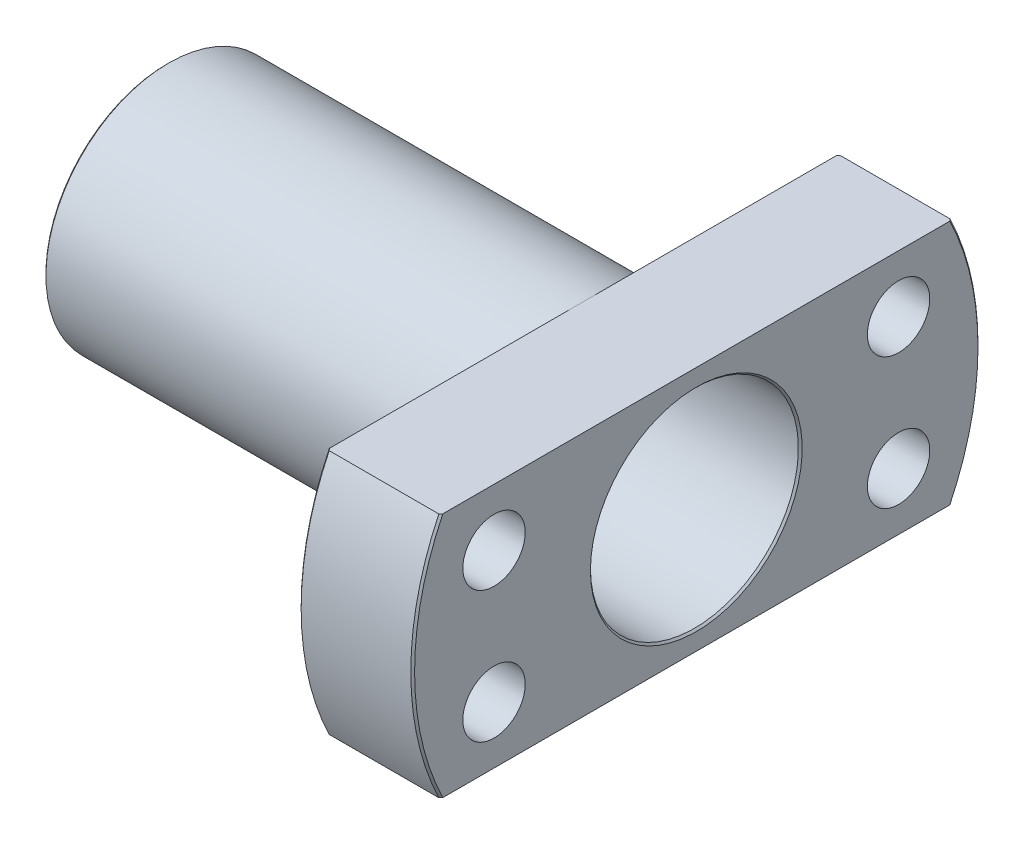
from build123d import *

# Parameters (mm, degrees)
SKETCH2_R                                           = 5.25
CUT_EXTRUDE1_DEPTH                                  = 71.256672281
CUT_EXTRUDE2_REACH                                  = 63.123
HOLE_SIZE_PER_HEX_SOCKET_HEAD_CAP_SCREW_D           = 6.6
HOLE_SIZE_PER_HEX_SOCKET_HEAD_CAP_SCREW_CBORE_D     = 11
HOLE_SIZE_PER_HEX_SOCKET_HEAD_CAP_SCREW_CBORE_DEPTH = 6.8
CHAMFER1_SIZE                                       = 0.2
CHAMFER2_SIZE                                       = 0.2
CHAMFER3_SIZE                                       = 1


with BuildPart() as part:
    # Sketch1 → Revolve1 (revolve)
    with BuildSketch(Plane.XY, mode=Mode.PRIVATE) as revolve1_sk:
        Polygon((0, 0), (0, 13), (44, 13), (44, 30), (56, 30), (56, 11), (6, 11), (6, 0), align=None)
    revolve(revolve1_sk.sketch.rotate(Axis((0, 0, 0), (1, 0, 0)), 90), axis=Axis((0, 0, 0), (1, 0, 0)))

    # Sketch2 → Cut-Extrude1 (cut, through all)
    with BuildSketch(Plane.ZY):
        Circle(SKETCH2_R)
    extrude(amount=-CUT_EXTRUDE1_DEPTH, mode=Mode.SUBTRACT)

    # Sketch3 → Cut-Extrude2 (cut, up to next)
    with BuildSketch(Plane.ZY.offset(-44), mode=Mode.PRIVATE) as cut_extrude2_sk1:
        with BuildLine():
            Line((27.037011669, 13), (-27.037011669, 13))
            ThreePointArc((-27.037011669, 13), (0, 30), (27.037011669, 13))
        make_face()
    cut_extrude2_tool1 = extrude(cut_extrude2_sk1.sketch, amount=-CUT_EXTRUDE2_REACH, mode=Mode.PRIVATE) & part.part
    # Sketch3 → Cut-Extrude2 (cut, up to next)
    with BuildSketch(Plane.ZY.offset(-44), mode=Mode.PRIVATE) as cut_extrude2_sk2:
        with BuildLine():
            Line((27.037011669, -13), (-27.037011669, -13))
            ThreePointArc((-27.037011669, -13), (0, -30), (27.037011669, -13))
        make_face()
    cut_extrude2_tool2 = extrude(cut_extrude2_sk2.sketch, amount=-CUT_EXTRUDE2_REACH, mode=Mode.PRIVATE) & part.part
    add(cut_extrude2_tool1.solids().sort_by_distance((44, 19.998046, 0))[0], mode=Mode.SUBTRACT)
    add(cut_extrude2_tool2.solids().sort_by_distance((44, -19.998046, 0))[0], mode=Mode.SUBTRACT)

    # Hole size per hex socket head cap screw type 1 (through all)
    with Locations(Plane(origin=(44, -6.952882373, 21.398771617), x_dir=(0, 0, -1), z_dir=(-1, 0, 0))):
        with Locations((0, 0), (0, -13.905764746), (42.797543234, -13.905764746), (42.797543234, 0)):
            CounterBoreHole(HOLE_SIZE_PER_HEX_SOCKET_HEAD_CAP_SCREW_D / 2, HOLE_SIZE_PER_HEX_SOCKET_HEAD_CAP_SCREW_CBORE_D / 2, HOLE_SIZE_PER_HEX_SOCKET_HEAD_CAP_SCREW_CBORE_DEPTH)

    # Chamfer1
    chamfer1_edges = [part.edges().sort_by_distance(p)[0] for p in [
        (0, 0, -5.25),
        (56, 0, 30),
        (44, 0, 30),
        (56, 0, -30),
        (44, 0, -30),
        (0, 0, -13),
    ]]
    chamfer(chamfer1_edges, length=CHAMFER1_SIZE)

    # Chamfer2
    chamfer2_edges = [part.edges().sort_by_distance(p)[0] for p in [
        (56, 0, -11),
    ]]
    chamfer(chamfer2_edges, length=CHAMFER2_SIZE)

    # Chamfer3
    chamfer3_edges = [part.edges().sort_by_distance(p)[0] for p in [
        (6, 0, -5.25),
    ]]
    chamfer(chamfer3_edges, length=CHAMFER3_SIZE)


solid = part.part
